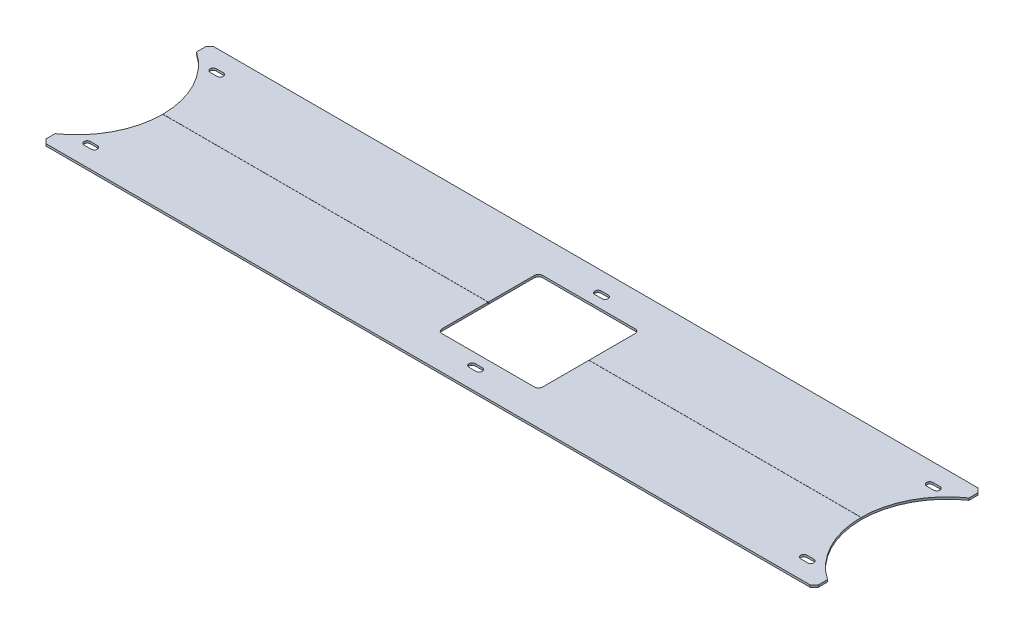
from build123d import *

# Parameters (mm, degrees)
SKETCH1_W           = 552
SKETCH1_H           = 120
BOSS_EXTRUDE1_DEPTH = 1.5
CHAMFER1_SIZE       = 3
CHAMFER2_SIZE       = 3
CUT_EXTRUDE6_DEPTH  = 283.45043813
SKETCH13_W          = 552
SKETCH13_H          = 0.1
CUT_EXTRUDE7_DEPTH  = 283.45043813
CUT_EXTRUDE9_DEPTH  = 283.45043813
SKETCH16_R          = 61.5
CUT_EXTRUDE10_DEPTH = 10
CUT_EXTRUDE11_DEPTH = 10


with BuildPart() as part:
    # Sketch1 → Boss-Extrude1 (new body)
    with BuildSketch(Plane(origin=(0, 0, 0), x_dir=(1, 0, 0), z_dir=(0, 1, 0))):
        Rectangle(SKETCH1_W, SKETCH1_H)
    extrude(amount=BOSS_EXTRUDE1_DEPTH)

    # Chamfer1
    chamfer1_edges = [part.edges().sort_by_distance(p)[0] for p in [
        (276, 0.75, 60),
        (276, 0.75, -60),
    ]]
    chamfer(chamfer1_edges, length=CHAMFER1_SIZE)

    # Chamfer2
    chamfer2_edges = [part.edges().sort_by_distance(p)[0] for p in [
        (-276, 0.75, 60),
        (-276, 0.75, -60),
    ]]
    chamfer(chamfer2_edges, length=CHAMFER2_SIZE)

    # Sketch12 → Cut-Extrude6 (cut, through all)
    with BuildSketch(Plane(origin=(0, 1.5, 0), x_dir=(1, 0, 0), z_dir=(0, 1, 0))):
        with BuildLine():
            Line((-258.5, 47.25), (-253.5, 47.25))
            ThreePointArc((-253.5, 47.25), (-251.25, 45), (-253.5, 42.75))
            Line((-253.5, 42.75), (-258.5, 42.75))
            ThreePointArc((-258.5, 42.75), (-260.75, 45), (-258.5, 47.25))
        make_face()
        with BuildLine():
            Line((-258.5, -42.75), (-253.5, -42.75))
            ThreePointArc((-253.5, -42.75), (-251.25, -45), (-253.5, -47.25))
            Line((-253.5, -47.25), (-258.5, -47.25))
            ThreePointArc((-258.5, -47.25), (-260.75, -45), (-258.5, -42.75))
        make_face()
    cut_extrude6 = extrude(amount=-CUT_EXTRUDE6_DEPTH, mode=Mode.SUBTRACT)

    # Sketch13 → Cut-Extrude7 (cut, through all)
    with BuildSketch(Plane(origin=(0, 1.5, 0), x_dir=(1, 0, 0), z_dir=(0, 1, 0))):
        Rectangle(SKETCH13_W, SKETCH13_H)
    extrude(amount=-CUT_EXTRUDE7_DEPTH, mode=Mode.SUBTRACT)


with BuildPart() as cut_extrude7_piece_1:
    # of the separate pieces the step leaves, piece 1, a body of its own (cut_extrude7_pieces)
    add(part.part.solids().sort_by_distance((-273, 0, -60))[0])


with BuildPart() as cut_extrude7_piece_2:
    # of the separate pieces the step leaves, piece 2, a body of its own (cut_extrude7_pieces)
    add(part.part.solids().sort_by_distance((-276, 0, 57))[0])


with BuildPart() as cut_extrude9_tool:
    # Sketch15 → Cut-Extrude9 (new, through all)
    with BuildSketch(Plane(origin=(0, 1.5, 0), x_dir=(1, 0, 0), z_dir=(0, 1, 0))):
        with BuildLine():
            Line((52, 35.95), (-14, 35.95))
            ThreePointArc((-14, 35.95), (-16.121320344, 35.071320344), (-17, 32.95))
            Line((-17, 32.95), (-17, -33.05))
            ThreePointArc((-17, -33.05), (-16.121320344, -35.171320344), (-14, -36.05))
            Line((-14, -36.05), (52, -36.05))
            ThreePointArc((52, -36.05), (54.121320344, -35.171320344), (55, -33.05))
            Line((55, -33.05), (55, 32.95))
            ThreePointArc((55, 32.95), (54.121320344, 35.071320344), (52, 35.95))
        make_face()
    extrude(amount=-CUT_EXTRUDE9_DEPTH)


with BuildPart() as cut_extrude7_piece_1_1:
    add(cut_extrude7_piece_1.part)

    # Cut-Extrude9: cut by cut_extrude9_tool
    add(cut_extrude9_tool.part, mode=Mode.SUBTRACT)


with BuildPart() as cut_extrude7_piece_2_1:
    add(cut_extrude7_piece_2.part)

    # Cut-Extrude9: cut by cut_extrude9_tool
    add(cut_extrude9_tool.part, mode=Mode.SUBTRACT)


with BuildPart() as cut_extrude10_tool:
    # Sketch16 → Cut-Extrude10 (new body)
    with BuildSketch(Plane(origin=(0, 1.5, 0), x_dir=(1, 0, 0), z_dir=(0, 1, 0))):
        with Locations((311, 0)):
            Circle(SKETCH16_R)
        with Locations((-311, 0)):
            Circle(SKETCH16_R)
    extrude(amount=-CUT_EXTRUDE10_DEPTH)


with BuildPart() as cut_extrude7_piece_1_2:
    add(cut_extrude7_piece_1_1.part)

    # Cut-Extrude10: cut by cut_extrude10_tool
    add(cut_extrude10_tool.part, mode=Mode.SUBTRACT)


with BuildPart() as cut_extrude7_piece_2_2:
    add(cut_extrude7_piece_2_1.part)

    # Cut-Extrude10: cut by cut_extrude10_tool
    add(cut_extrude10_tool.part, mode=Mode.SUBTRACT)


with BuildPart() as mirror1_tool:
    # Mirror1: Cut-Extrude6 across plane
    add(cut_extrude6.mirror(Plane(origin=(0, 0, 0), x_dir=(0, 0, 1), z_dir=(1, 0, 0))))


with BuildPart() as cut_extrude7_piece_1_3:
    add(cut_extrude7_piece_1_2.part)

    # Mirror1: cut by mirror1_tool
    add(mirror1_tool.part, mode=Mode.SUBTRACT)


with BuildPart() as cut_extrude7_piece_2_3:
    add(cut_extrude7_piece_2_2.part)

    # Mirror1: cut by mirror1_tool
    add(mirror1_tool.part, mode=Mode.SUBTRACT)


with BuildPart() as cut_extrude11_tool:
    # Sketch17 → Cut-Extrude11 (new body)
    with BuildSketch(Plane.XZ):
        with BuildLine():
            Line((21.5, -47.25), (16.5, -47.25))
            ThreePointArc((16.5, -47.25), (14.25, -45), (16.5, -42.75))
            Line((16.5, -42.75), (21.5, -42.75))
            ThreePointArc((21.5, -42.75), (23.75, -45), (21.5, -47.25))
        make_face()
        with BuildLine():
            Line((21.5, 42.75), (16.5, 42.75))
            ThreePointArc((16.5, 42.75), (14.25, 45), (16.5, 47.25))
            Line((16.5, 47.25), (21.5, 47.25))
            ThreePointArc((21.5, 47.25), (23.75, 45), (21.5, 42.75))
        make_face()
    extrude(amount=-CUT_EXTRUDE11_DEPTH)


with BuildPart() as cut_extrude7_piece_1_4:
    add(cut_extrude7_piece_1_3.part)

    # Cut-Extrude11: cut by cut_extrude11_tool
    add(cut_extrude11_tool.part, mode=Mode.SUBTRACT)


with BuildPart() as cut_extrude7_piece_2_4:
    add(cut_extrude7_piece_2_3.part)

    # Cut-Extrude11: cut by cut_extrude11_tool
    add(cut_extrude11_tool.part, mode=Mode.SUBTRACT)


solid = Compound([cut_extrude7_piece_1_4.part, cut_extrude7_piece_2_4.part])
